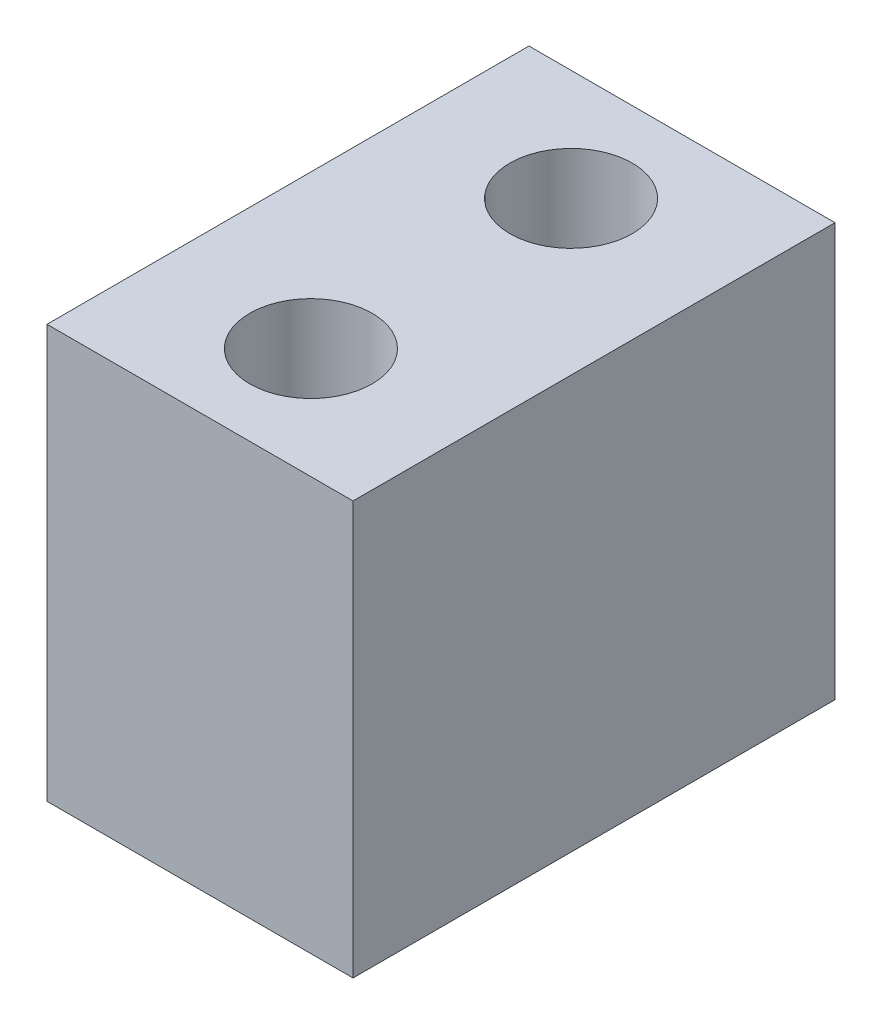
SolidWorks part; units mm, degrees
material "Q235"
ref_plane "Front Plane" through (0, 0, 0) normal (0, 0, 1) x (1, 0, 0)
ref_plane "Top Plane" through (0, 0, 0) normal (0, 1, 0) x (1, 0, 0)
ref_plane "Right Plane" through (0, 0, 0) normal (1, 0, 0) x (0, 0, -1)
sketch "Sketch2" plane through (0, 0, 0) normal (0, 1, 0) x (1, 0, 0)
  line L0 (-131.395, 0) -> (113.7022, 0) construction
  line L1 (0, 164.1787) -> (0, -121.5078) construction
  line L3 (-40, 63) -> (40, 63)
  line L4 (-40, 63) -> (-40, -63)
  line L5 (-40, -63) -> (40, -63)
  line L6 (40, 63) -> (40, -63)
  dimension "D1" = 126
  dimension "D2" = 80
  dimension "D3" = 40
extrude "Boss-Extrude1" add sketch "Sketch2" along normal mid plane 108
hole_wizard "M36 Tapped Hole1" positions "Sketch4" profile "Sketch3" tap size "M36" standard "GB"
sketch "Sketch4" plane through (0, 54, 0) normal (0, 1, 0) x (1, 0, 0)
  line L0 (0, 87.994) -> (0, -83.4139) construction
  line L2 (-50.2782, 0) -> (51.8371, 0) construction
  point P0 (0, 34)
  point P3 (0, -34)
  dimension "D1" = 68
cosmetic thread "Cosmetic Thread1" parameters "D1"=60, "D2"=36
cosmetic thread "Cosmetic Thread2" parameters "D1"=60, "D2"=36
sketch "Sketch3" plane through (0, 54, -34) normal (1, 0, 0) x (0, 0, 1)
  line L0 (0, 0) -> (0, 89.6138)
  line L1 (0, 89.6138) -> (16, 80)
  line L2 (16, 80) -> (16, 0)
  line L5 (16, 0) -> (0, 0)
  line L10 (0, 89.6138) -> (-16, 80) construction
  line L11 (0, -6.35) -> (0, 107.95) construction
  dimension "螺纹孔钻头直径" = 32
  dimension "螺纹孔钻头深度" = 80
  dimension "导头角度" = 118
